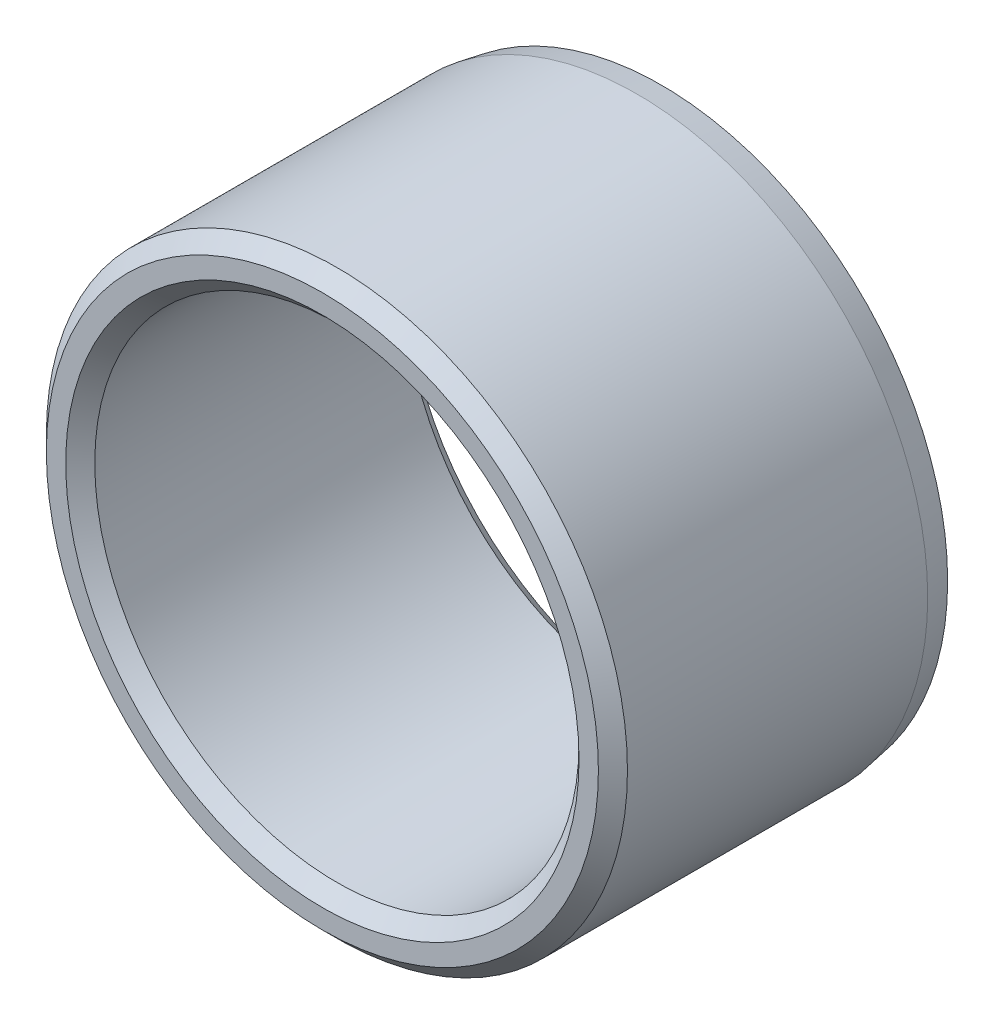
from build123d import *

# Parameters (mm, degrees)
SKETCH1_R           = 60
SKETCH1_R_2         = 50
BOSS_EXTRUDE1_DEPTH = 35
CHAMFER1_SIZE       = 3
CHAMFER2_SIZE       = 5
CHAMFER2_SIZE2      = 0.881634904


with BuildPart() as part:
    # Sketch1 → Boss-Extrude1 (new, symmetric)
    with BuildSketch(Plane.XY):
        Circle(SKETCH1_R)
        Circle(SKETCH1_R_2, mode=Mode.SUBTRACT)
    extrude(amount=BOSS_EXTRUDE1_DEPTH, both=True)

    # Chamfer1
    chamfer1_edges = [part.edges().sort_by_distance(p)[0] for p in [
        (-60, 0, 35),
        (-50, 0, -35),
        (-50, 0, 35),
    ]]
    chamfer(chamfer1_edges, length=CHAMFER1_SIZE)

    # Chamfer2
    chamfer2_edges = [part.edges().sort_by_distance(p)[0] for p in [
        (-60, 0, -35),
    ]]
    chamfer2_side = [part.faces().sort_by_distance(p)[0] for p in [
        (-60, 0, -1.5),
    ]]
    chamfer(chamfer2_edges, length=CHAMFER2_SIZE, length2=CHAMFER2_SIZE2, reference=chamfer2_side[0])


solid = part.part
